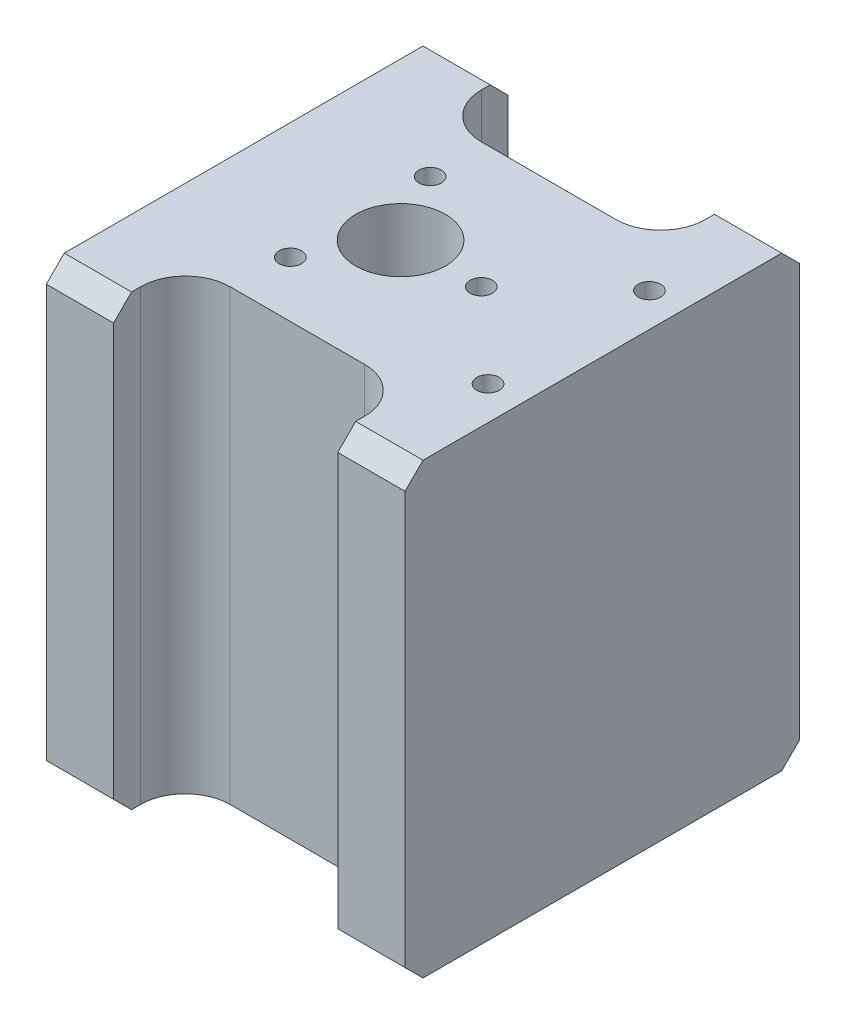
from build123d import *

# Parameters (mm, degrees)
SKETCH1_W             = 40
SKETCH1_H             = 50
BOSS_EXTRUDE1_DEPTH   = 44
SKETCH2_R             = 5
CUT_EXTRUDE1_DEPTH    = 20
CIRPATTERN1_COUNT     = 3
M4_TAPPED_HOLE1_D     = 3.3
M4_TAPPED_HOLE1_DEPTH = 10.1
M4_TAPPED_HOLE1_TIP   = 0.991420021
SKETCH7_W             = 25
SKETCH7_H             = 8
CUT_EXTRUDE2_DEPTH    = 70.541354603
CHAMFER1_SIZE         = 2
FILLET1_R             = 5
M3_TAPPED_HOLE2_D     = 2.5
M3_TAPPED_HOLE2_DEPTH = 8.5
M3_TAPPED_HOLE2_TIP   = 0.751075774


with BuildPart() as part:
    # Sketch1 → Boss-Extrude1 (new body)
    with BuildSketch(Plane.XY):
        Rectangle(SKETCH1_W, SKETCH1_H)
    extrude(amount=BOSS_EXTRUDE1_DEPTH)

    # Sketch2 → Cut-Extrude1 (cut)
    with BuildSketch(Plane(origin=(0, 25, 0), x_dir=(1, 0, 0), z_dir=(0, 1, 0))):
        with Locations(Location((-2.5, -22, 0), (0, 0, 270))):
            Circle(SKETCH2_R)
    extrude(amount=-CUT_EXTRUDE1_DEPTH, mode=Mode.SUBTRACT)

    # Sketch3 → M3 Tapped Hole1 (revolve, cut)
    with BuildSketch(Plane(origin=(6.5, 25, 22), x_dir=(0, 0, 1), z_dir=(1, 0, 0))):
        Polygon((0, 0), (0, 8.251075774), (1.25, 7.5), (1.25, 0), align=None)
    m3_tapped_hole1 = revolve(axis=Axis((6.5, 31.35, 22), (0, -1, 0)), mode=Mode.SUBTRACT)

    # CirPattern1: M3 Tapped Hole1 ×3 about axis
    cirpattern1_axis = Axis((-2.5, 0, 22), (0, 1, 0))
    for i in range(1, CIRPATTERN1_COUNT):
        add(m3_tapped_hole1.rotate(cirpattern1_axis, i * 360 / CIRPATTERN1_COUNT), mode=Mode.SUBTRACT)

    # M4 Tapped Hole1
    with Locations(Plane(origin=(0, -25, 0), x_dir=(-1, 0, 0), z_dir=(0, -1, 0))):
        with Locations((-14, -32), (2, -32), (-14, -12), (2, -12)):
            Hole(M4_TAPPED_HOLE1_D / 2, depth=M4_TAPPED_HOLE1_DEPTH)
            with Locations((0, 0, -(M4_TAPPED_HOLE1_DEPTH + M4_TAPPED_HOLE1_TIP / 2))):  # 118° drill point
                Cone(0, M4_TAPPED_HOLE1_D / 2, M4_TAPPED_HOLE1_TIP, mode=Mode.SUBTRACT)

    # Sketch7 → Cut-Extrude2 (cut, through all)
    with BuildSketch(Plane.XZ.offset(25)):
        with Locations((0, 40)):
            Rectangle(SKETCH7_W, SKETCH7_H)
        with Locations((0, 4)):
            Rectangle(SKETCH7_W, SKETCH7_H)
    extrude(amount=-CUT_EXTRUDE2_DEPTH, mode=Mode.SUBTRACT)

    # Chamfer1
    chamfer1_edges = [part.edges().sort_by_distance(p)[0] for p in [
        (-16.25, -25, 44),
        (-16.25, -25, 0),
        (-16.25, 25, 44),
        (16.25, -25, 44),
        (16.25, 25, 0),
        (16.25, -25, 0),
        (-16.25, 25, 0),
        (16.25, 25, 44),
    ]]
    chamfer(chamfer1_edges, length=CHAMFER1_SIZE)

    # Fillet1
    fillet1_edges = [part.edges().sort_by_distance(p)[0] for p in [
        (12.5, 0, 36),
        (-12.5, 0, 36),
        (12.5, 0, 8),
        (-12.5, 0, 8),
    ]]
    fillet(fillet1_edges, radius=FILLET1_R)

    # M3 Tapped Hole2
    with Locations(Plane(origin=(0, 25, 0), x_dir=(1, 0, 0), z_dir=(0, 1, 0))):
        with Locations((16.25, -31), (16.25, -13)):
            Hole(M3_TAPPED_HOLE2_D / 2, depth=M3_TAPPED_HOLE2_DEPTH)
            with Locations((0, 0, -(M3_TAPPED_HOLE2_DEPTH + M3_TAPPED_HOLE2_TIP / 2))):  # 118° drill point
                Cone(0, M3_TAPPED_HOLE2_D / 2, M3_TAPPED_HOLE2_TIP, mode=Mode.SUBTRACT)


solid = part.part
